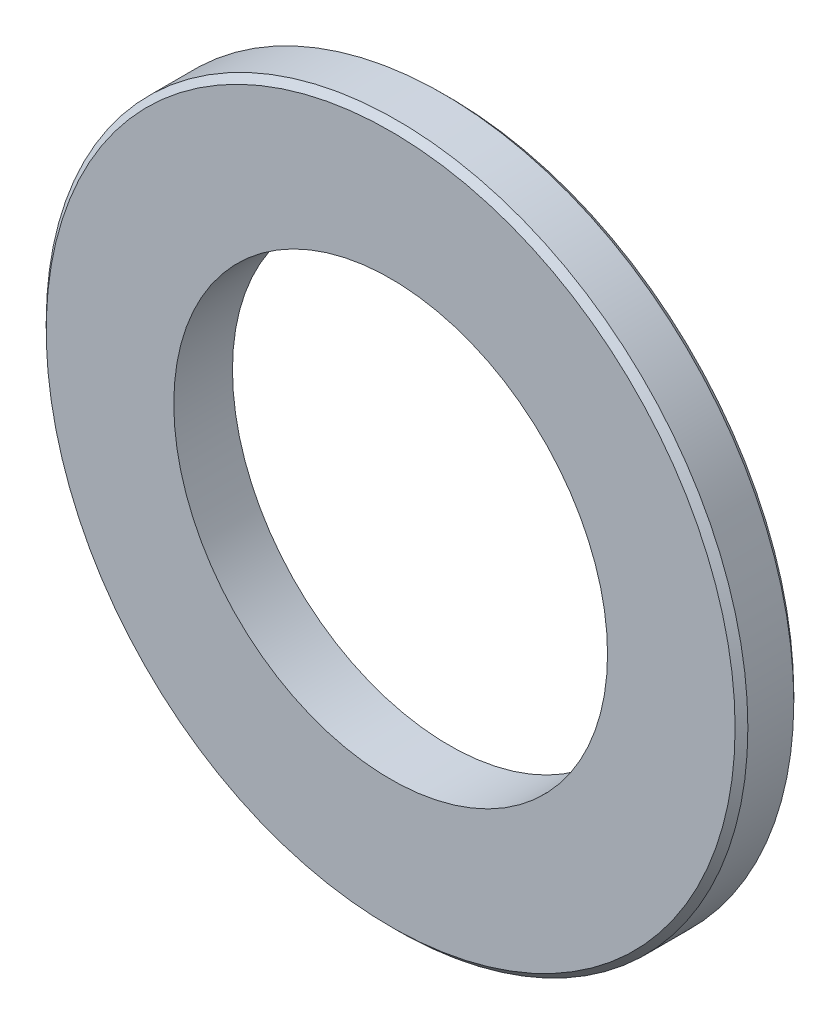
from build123d import *

# Parameters (mm, degrees)
SKETCH_1_R      = 27.5
SKETCH_1_R_2    = 17
EXTRUDE_1_DEPTH = 4.6
CHAMFER_1_SIZE  = 0.5


with BuildPart() as part:
    # 草图1 → 凸台-拉伸1 (new body)
    with BuildSketch(Plane.XY):
        Circle(SKETCH_1_R)
        Circle(SKETCH_1_R_2, mode=Mode.SUBTRACT)
    extrude(amount=EXTRUDE_1_DEPTH)

    # 倒角1
    chamfer_1_edges = [part.edges().sort_by_distance(p)[0] for p in [
        (-27.5, 0, 0),
        (-27.5, 0, 4.6),
    ]]
    chamfer(chamfer_1_edges, length=CHAMFER_1_SIZE)


solid = part.part
